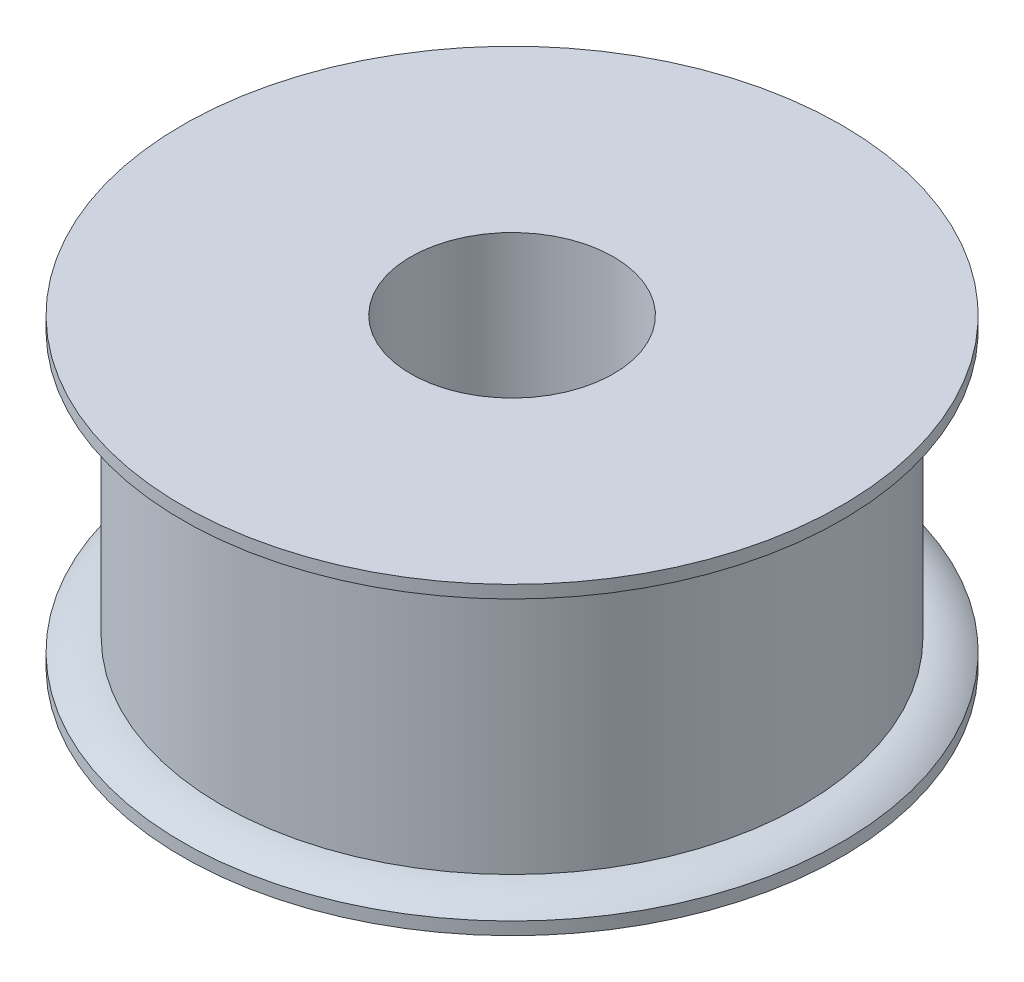
from build123d import *


with BuildPart() as part:
    # Sketch1 → Revolve1 (revolve)
    with BuildSketch(Plane.XY, mode=Mode.PRIVATE) as revolve1_sk:
        Polygon((11.46, -5), (11.46, 5), (8, 5), (8, 6), (4, 6), (4, -6), (8, -6), (8, -5), align=None)
    revolve(revolve1_sk.sketch.rotate(Axis((0, 0, 0), (0, 1, 0)), 90), axis=Axis((0, 0, 0), (0, 1, 0)))

    # Sketch2 → Revolve2 (revolve)
    with BuildSketch(Plane.XY, mode=Mode.PRIVATE) as revolve2_sk:
        with BuildLine():
            Line((8, 5), (11.46, 5))
            ThreePointArc((11.46, 5), (12.269567786, 5.128131219), (13, 5.5))
            Line((13, 5.5), (13, 6))
            Line((13, 6), (8, 6))
            Line((8, 6), (8, 5))
        make_face()
        with BuildLine():
            Line((13, -5.5), (13, -6))
            Line((13, -6), (8, -6))
            Line((8, -6), (8, -5))
            Line((8, -5), (11.46, -5))
            ThreePointArc((11.46, -5), (12.269567786, -5.128131219), (13, -5.5))
        make_face()
    revolve(revolve2_sk.sketch.rotate(Axis((0, 0, 0), (0, 1, 0)), 90), axis=Axis((0, 0, 0), (0, 1, 0)))


solid = part.part
